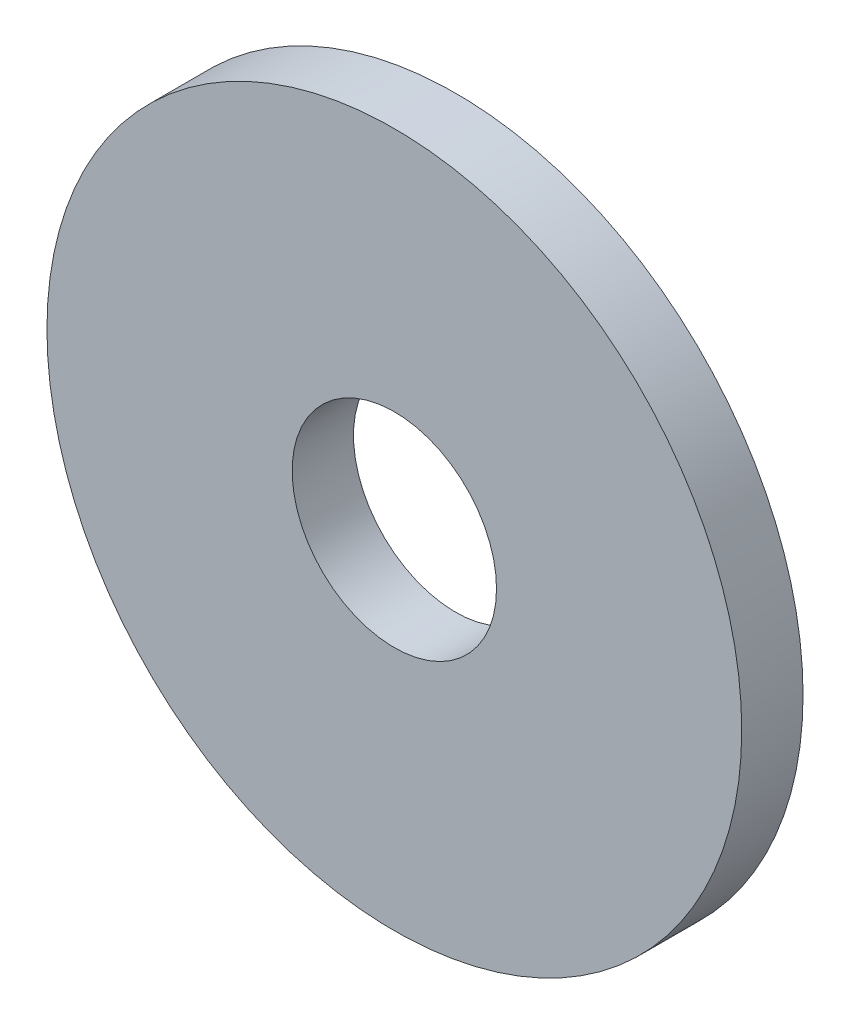
SolidWorks part; units mm, degrees
ref_plane "Front Plane" through (0, 0, 0) normal (0, 0, 1) x (1, 0, 0)
ref_plane "Top Plane" through (0, 0, 0) normal (0, 1, 0) x (1, 0, 0)
ref_plane "Right Plane" through (0, 0, 0) normal (1, 0, 0) x (0, 0, -1)
other "Configuration Table"
sketch "Sketch1" plane through (0, 0, 0) normal (0, 0, 1) x (1, 0, 0)
  circle A0 centre (0, 0) radius 85
  circle A1 centre (0, 0) radius 25
extrude "Boss-Extrude1" add sketch "Sketch1" along normal blind 15
